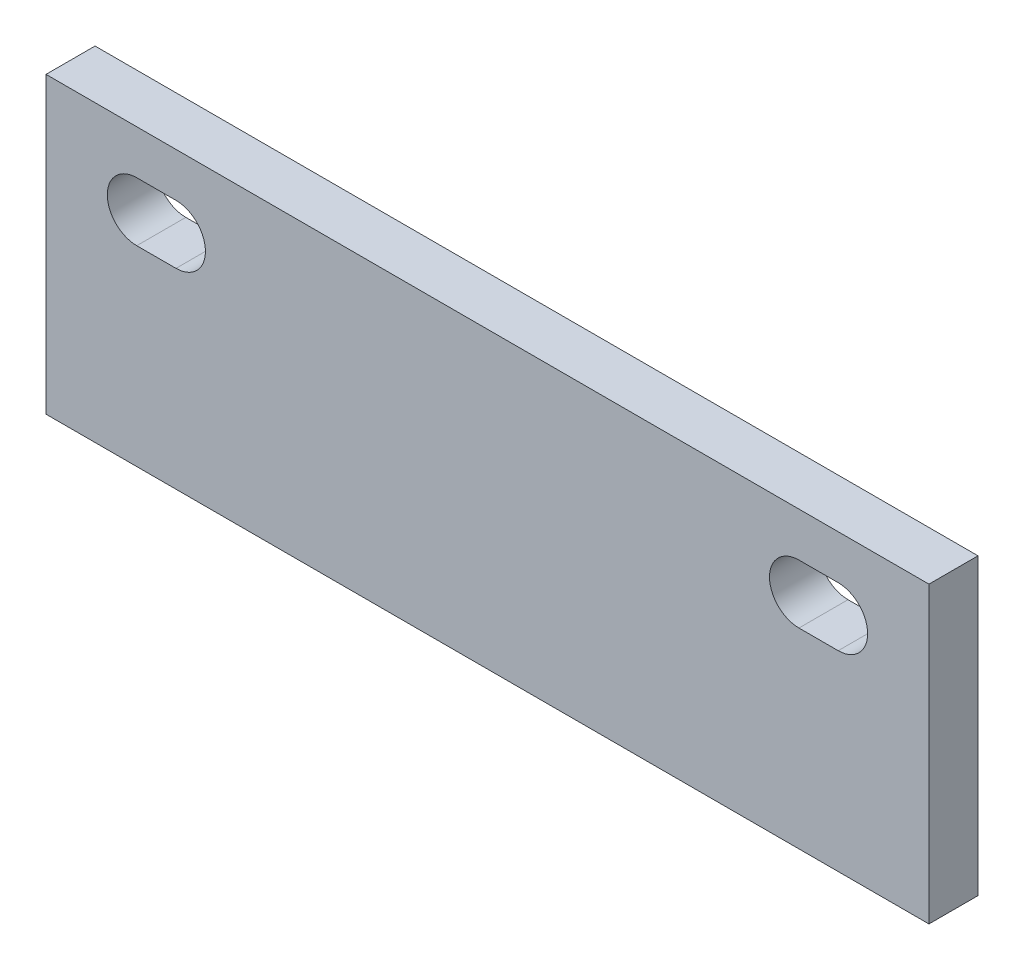
from build123d import *

# Parameters (mm, degrees)
SKETCH_1_W      = 180
SKETCH_1_H      = 60
EXTRUDE_1_DEPTH = 10


with BuildPart() as part:
    # 草图1 → 凸台-拉伸1 (new body)
    with BuildSketch(Plane.XY):
        Rectangle(SKETCH_1_W, SKETCH_1_H)
        with BuildLine():
            Line((-71.5, 21), (-63.5, 21))
            ThreePointArc((-63.5, 21), (-57.5, 15), (-63.5, 9))
            Line((-63.5, 9), (-71.5, 9))
            ThreePointArc((-71.5, 9), (-77.5, 15), (-71.5, 21))
        make_face(mode=Mode.SUBTRACT)
        with BuildLine():
            Line((63.5, 21), (71.5, 21))
            ThreePointArc((71.5, 21), (77.5, 15), (71.5, 9))
            Line((71.5, 9), (63.5, 9))
            ThreePointArc((63.5, 9), (57.5, 15), (63.5, 21))
        make_face(mode=Mode.SUBTRACT)
    extrude(amount=EXTRUDE_1_DEPTH)


solid = part.part
